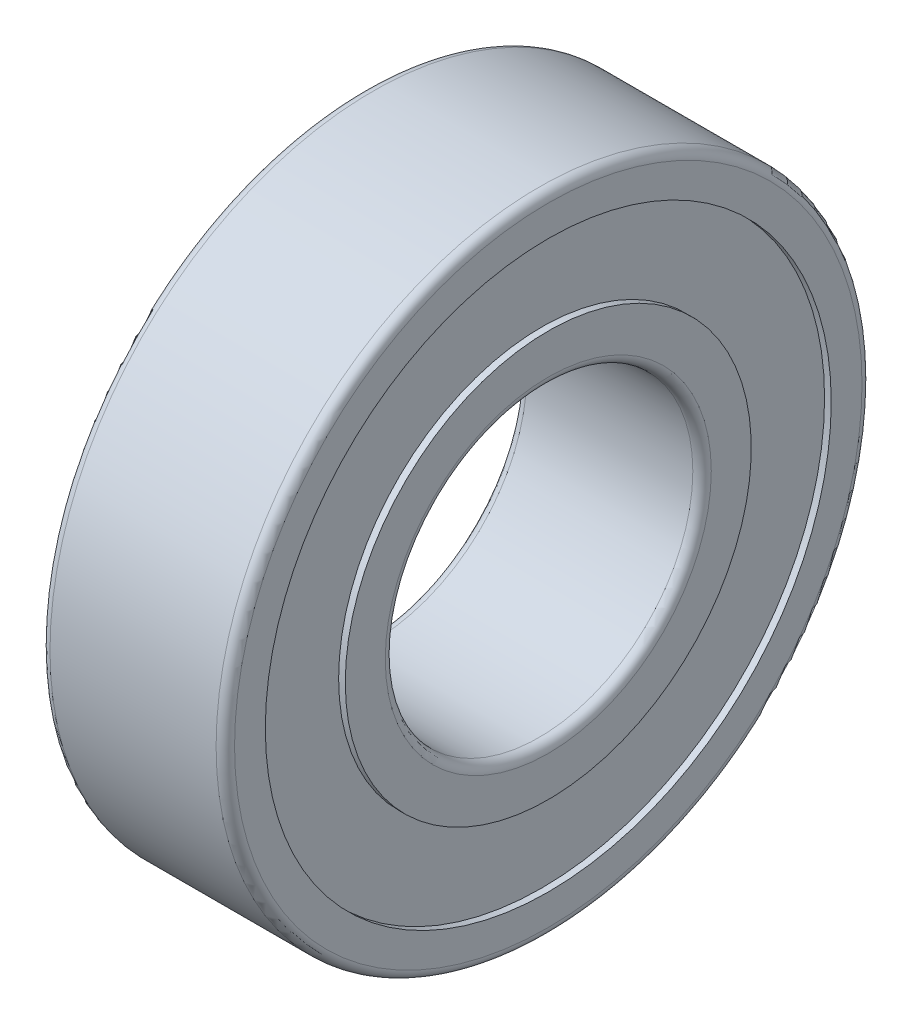
from build123d import *


with BuildPart() as part:
    # 草图1 → 旋转1 (revolve)
    with BuildSketch(Plane.XY, mode=Mode.PRIVATE) as revolve_1_sk:
        with BuildLine():
            Line((0, 20.4), (0, 18.4))
            Line((0, 18.4), (0.433, 18.4))
            Line((0.433, 18.4), (0.433, 13.2))
            Line((0.433, 13.2), (0, 13.2))
            Line((0, 13.2), (0, 10.6))
            ThreePointArc((0, 10.6), (0.175735931, 10.175735931), (0.6, 10))
            Line((0.6, 10), (11.4, 10))
            ThreePointArc((11.4, 10), (11.824264069, 10.175735931), (12, 10.6))
            Line((12, 10.6), (12, 13.2))
            Line((12, 13.2), (11.567, 13.2))
            Line((11.567, 13.2), (11.567, 18.4))
            Line((11.567, 18.4), (12, 18.4))
            Line((12, 18.4), (12, 20.4))
            ThreePointArc((12, 20.4), (11.824264069, 20.824264069), (11.4, 21))
            Line((11.4, 21), (0.6, 21))
            ThreePointArc((0.6, 21), (0.175735931, 20.824264069), (0, 20.4))
        make_face()
    revolve(revolve_1_sk.sketch.rotate(Axis((12, 0, 0), (-1, 0, 0)), 270), axis=Axis((12, 0, 0), (-1, 0, 0)))


solid = part.part
